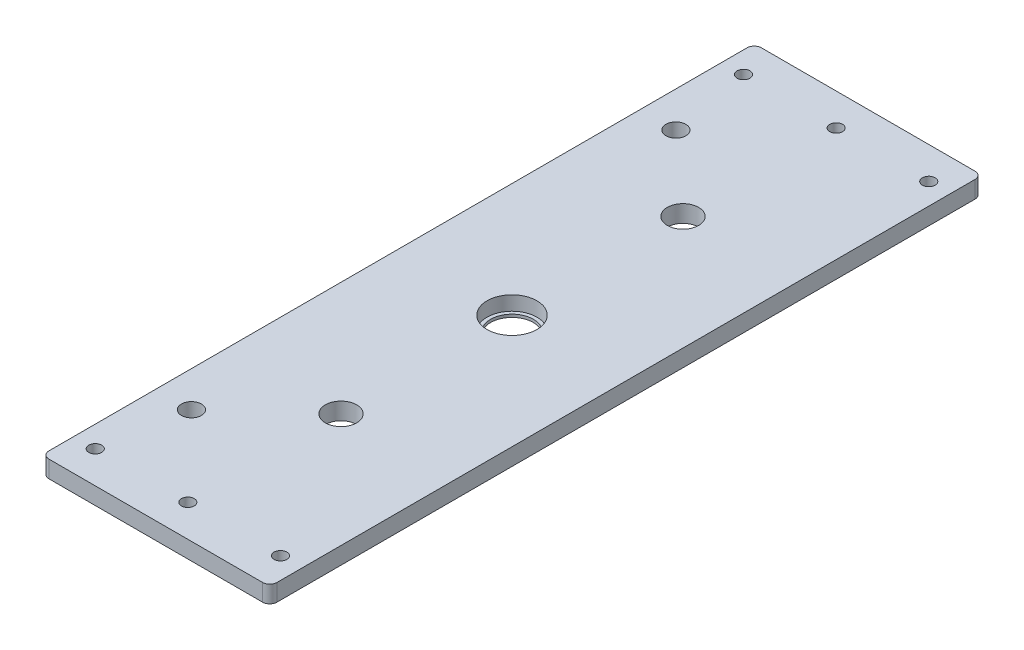
from build123d import *

# Parameters (mm, degrees)
SKETCH1_W                    = 160
SKETCH1_H                    = 500
BOSS_EXTRUDE1_DEPTH          = 12
SKETCH2_R                    = 15
SKETCH2_R_2                  = 11
CUT_EXTRUDE1_DEPTH           = 12
SKETCH3_R                    = 17.5
CUT_EXTRUDE2_DEPTH           = 10
F_9_0_9_DIAMETER_HOLE1_D     = 9
F_9_0_9_DIAMETER_HOLE1_DEPTH = 13
F_9_0_9_DIAMETER_HOLE1_TIP   = 2.703872786
FILLET1_R                    = 5
SKETCH7_R                    = 7
CUT_EXTRUDE3_DEPTH           = 263.762249952


with BuildPart() as part:
    # Sketch1 → Boss-Extrude1 (new body)
    with BuildSketch(Plane(origin=(0, 0, 0), x_dir=(1, 0, 0), z_dir=(0, 1, 0))):
        Rectangle(SKETCH1_W, SKETCH1_H)
    extrude(amount=BOSS_EXTRUDE1_DEPTH)

    # Sketch2 → Cut-Extrude1 (cut)
    with BuildSketch(Plane(origin=(0, 12, 0), x_dir=(1, 0, 0), z_dir=(0, 1, 0))):
        with Locations(Location((0, 0, 0), (0, 0, 270))):
            Circle(SKETCH2_R)
        with Locations(Location((0, -120, 0), (0, 0, 270))):
            Circle(SKETCH2_R_2)
        with Locations(Location((0, 120, 0), (0, 0, 90))):
            Circle(SKETCH2_R_2)
    extrude(amount=-CUT_EXTRUDE1_DEPTH, mode=Mode.SUBTRACT)

    # Sketch3 → Cut-Extrude2 (cut)
    with BuildSketch(Plane(origin=(0, 12, 0), x_dir=(1, 0, 0), z_dir=(0, 1, 0))):
        with Locations(Location((0, 0, 0), (0, 0, 270))):
            Circle(SKETCH3_R)
    extrude(amount=-CUT_EXTRUDE2_DEPTH, mode=Mode.SUBTRACT)

    # Ø9.0 (9) Diameter Hole1
    with Locations(Plane(origin=(0, 12, 0), x_dir=(1, 0, 0), z_dir=(0, 1, 0))):
        with Locations((-65, 227.5), (0, 227.5), (65, 227.5), (-65, -227.5), (0, -227.5), (65, -227.5)):
            Hole(F_9_0_9_DIAMETER_HOLE1_D / 2, depth=F_9_0_9_DIAMETER_HOLE1_DEPTH)
            with Locations((0, 0, -(F_9_0_9_DIAMETER_HOLE1_DEPTH + F_9_0_9_DIAMETER_HOLE1_TIP / 2))):  # 118° drill point
                Cone(0, F_9_0_9_DIAMETER_HOLE1_D / 2, F_9_0_9_DIAMETER_HOLE1_TIP, mode=Mode.SUBTRACT)

    # Fillet1
    fillet1_edges = [part.edges().sort_by_distance(p)[0] for p in [
        (80, 6, 250),
        (-80, 6, 250),
        (-80, 6, -250),
        (80, 6, -250),
    ]]
    fillet(fillet1_edges, radius=FILLET1_R)

    # Sketch7 → Cut-Extrude3 (cut, through all)
    with BuildSketch(Plane.XZ):
        with Locations(Location((-55, 170, 0), (0, 0, 270))):
            Circle(SKETCH7_R)
        with Locations(Location((-55, -170, 0), (0, 0, 90))):
            Circle(SKETCH7_R)
    extrude(amount=-CUT_EXTRUDE3_DEPTH, mode=Mode.SUBTRACT)


solid = part.part
